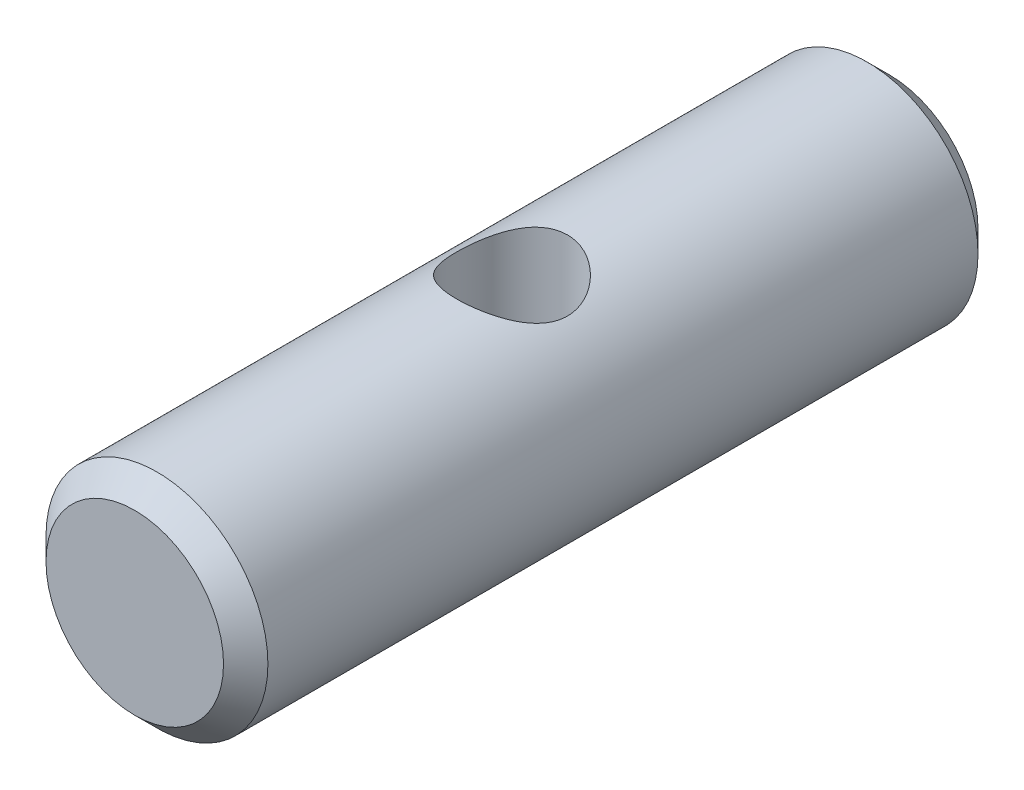
from build123d import *

# Parameters (mm, degrees)
SKETCH1_W                = 5
SKETCH1_H                = 34
F_5_0_5_DIAMETER_HOLE1_D = 5
CHAMFER1_SIZE            = 1


with BuildPart() as part:
    # Sketch1 → Revolve1 (revolve)
    with BuildSketch(Plane.XZ, mode=Mode.PRIVATE) as revolve1_sk:
        with Locations((2.5, 17)):
            Rectangle(SKETCH1_W, SKETCH1_H)
    revolve(revolve1_sk.sketch.rotate(Axis((0, 0, 34), (0, 0, -1)), 180), axis=Axis((0, 0, 34), (0, 0, -1)))

    # Ø5.0 (5) Diameter Hole1 (through all)
    with Locations(Plane(origin=(0, -5, 17), x_dir=(-1, 0, 0), z_dir=(0, -1, 0))):
        with Locations((0, 0)):
            Hole(F_5_0_5_DIAMETER_HOLE1_D / 2)

    # Chamfer1
    chamfer1_edges = [part.edges().sort_by_distance(p)[0] for p in [
        (5, 0, 0),
        (5, 0, 34),
    ]]
    chamfer(chamfer1_edges, length=CHAMFER1_SIZE)


solid = part.part
